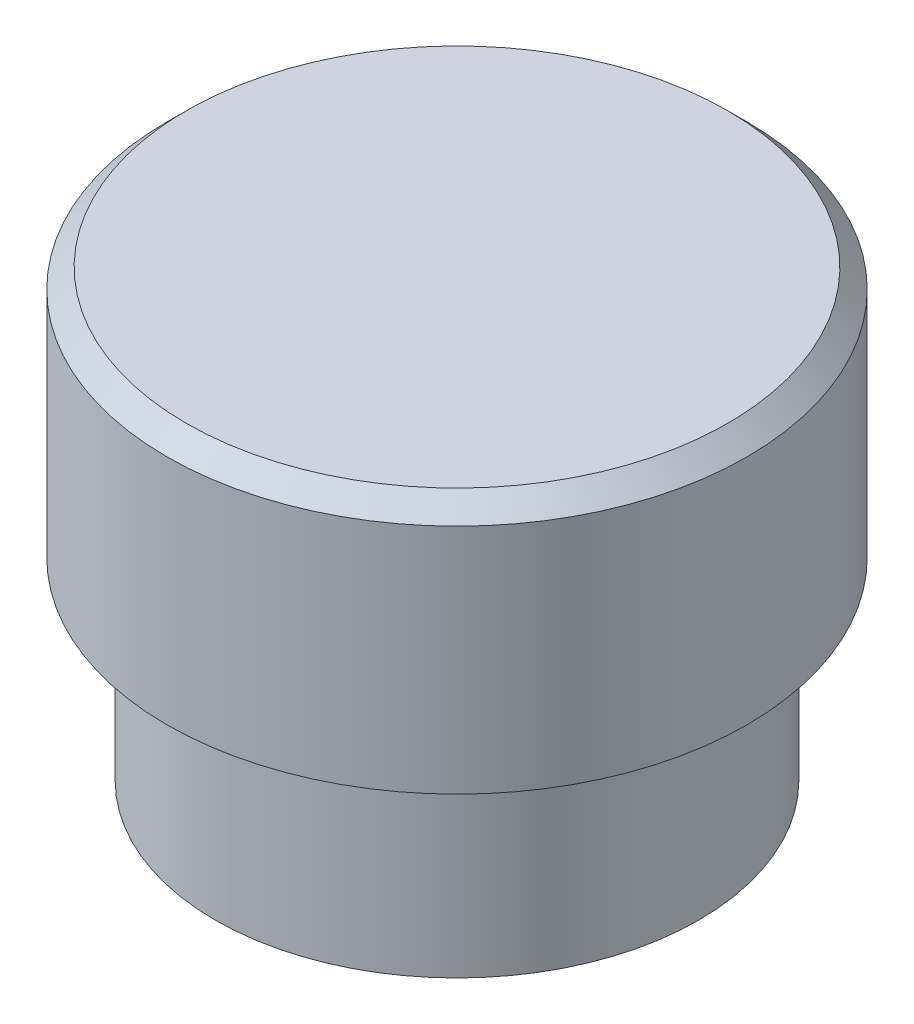
from build123d import *

# Parameters (mm, degrees)
SKETCH_1_R      = 15
EXTRUDE_1_DEPTH = 13
SKETCH_2_R      = 12.5
EXTRUDE_2_DEPTH = 10
CHAMFER_1_SIZE  = 1


with BuildPart() as part:
    # 草图1 → 凸台-拉伸1 (new body)
    with BuildSketch(Plane(origin=(0, 0, 0), x_dir=(1, 0, 0), z_dir=(0, 1, 0))):
        with Locations(Location((0, 0, 0), (0, 0, 90))):
            Circle(SKETCH_1_R)
    extrude(amount=EXTRUDE_1_DEPTH)

    # 草图2 → 凸台-拉伸2 (add)
    with BuildSketch(Plane.XZ):
        with Locations(Location((0, 0, 0), (0, 0, 270))):
            Circle(SKETCH_2_R)
    extrude(amount=EXTRUDE_2_DEPTH)

    # 倒角1
    chamfer_1_edges = [part.edges().sort_by_distance(p)[0] for p in [
        (0, 13, 15),
    ]]
    chamfer(chamfer_1_edges, length=CHAMFER_1_SIZE)


solid = part.part
